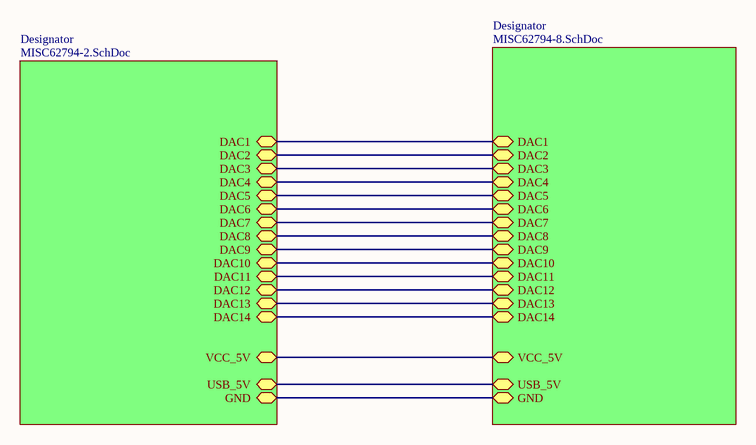
[diagram p0: MISC62794-10.SchDoc]
# Altium project MISC62794-12.PrjPcb (part 1 of 3)
3 sheets, 158 parts. Net scope: global (net labels, ports and power ports of the same name join across sheets).
Board file: MISC62794.PcbDoc
Sheets:
  MISC62794-10.SchDoc
    Designator = MISC62794-2.SchDoc
    Designator = MISC62794-8.SchDoc

## Sheet MISC62794-10.SchDoc
size A4

### Sub-sheets
Designator = MISC62794-2.SchDoc: DAC1 (bidir), DAC2 (bidir), DAC3 (bidir), DAC4 (bidir), DAC5 (bidir), DAC6 (bidir), DAC7 (bidir), DAC8 (bidir), DAC9 (bidir), DAC10 (bidir), DAC11 (bidir), DAC12 (bidir), DAC13 (bidir), DAC14 (bidir), USB_5V (bidir), GND (bidir), VCC_5V (bidir)
Designator = MISC62794-8.SchDoc: DAC1 (bidir), DAC2 (bidir), DAC3 (bidir), DAC4 (bidir), DAC5 (bidir), DAC6 (bidir), DAC7 (bidir), DAC8 (bidir), DAC9 (bidir), DAC10 (bidir), DAC11 (bidir), DAC12 (bidir), DAC13 (bidir), DAC14 (bidir), USB_5V (bidir), GND (bidir), VCC_5V (bidir)

### Nets
(unnamed): sheet Designator/DAC1, sheet Designator/DAC1
(unnamed): sheet Designator/DAC2, sheet Designator/DAC2
(unnamed): sheet Designator/DAC3, sheet Designator/DAC3
(unnamed): sheet Designator/DAC4, sheet Designator/DAC4
(unnamed): sheet Designator/DAC5, sheet Designator/DAC5
(unnamed): sheet Designator/DAC6, sheet Designator/DAC6
(unnamed): sheet Designator/DAC7, sheet Designator/DAC7
(unnamed): sheet Designator/DAC8, sheet Designator/DAC8
(unnamed): sheet Designator/DAC9, sheet Designator/DAC9
(unnamed): sheet Designator/DAC10, sheet Designator/DAC10
(unnamed): sheet Designator/DAC11, sheet Designator/DAC11
(unnamed): sheet Designator/DAC12, sheet Designator/DAC12
(unnamed): sheet Designator/DAC13, sheet Designator/DAC13
(unnamed): sheet Designator/DAC14, sheet Designator/DAC14
(unnamed): sheet Designator/USB_5V, sheet Designator/USB_5V
(unnamed): sheet Designator/GND, sheet Designator/GND
(unnamed): sheet Designator/VCC_5V, sheet Designator/VCC_5V

## Sheet MISC62794-2.SchDoc
size A4
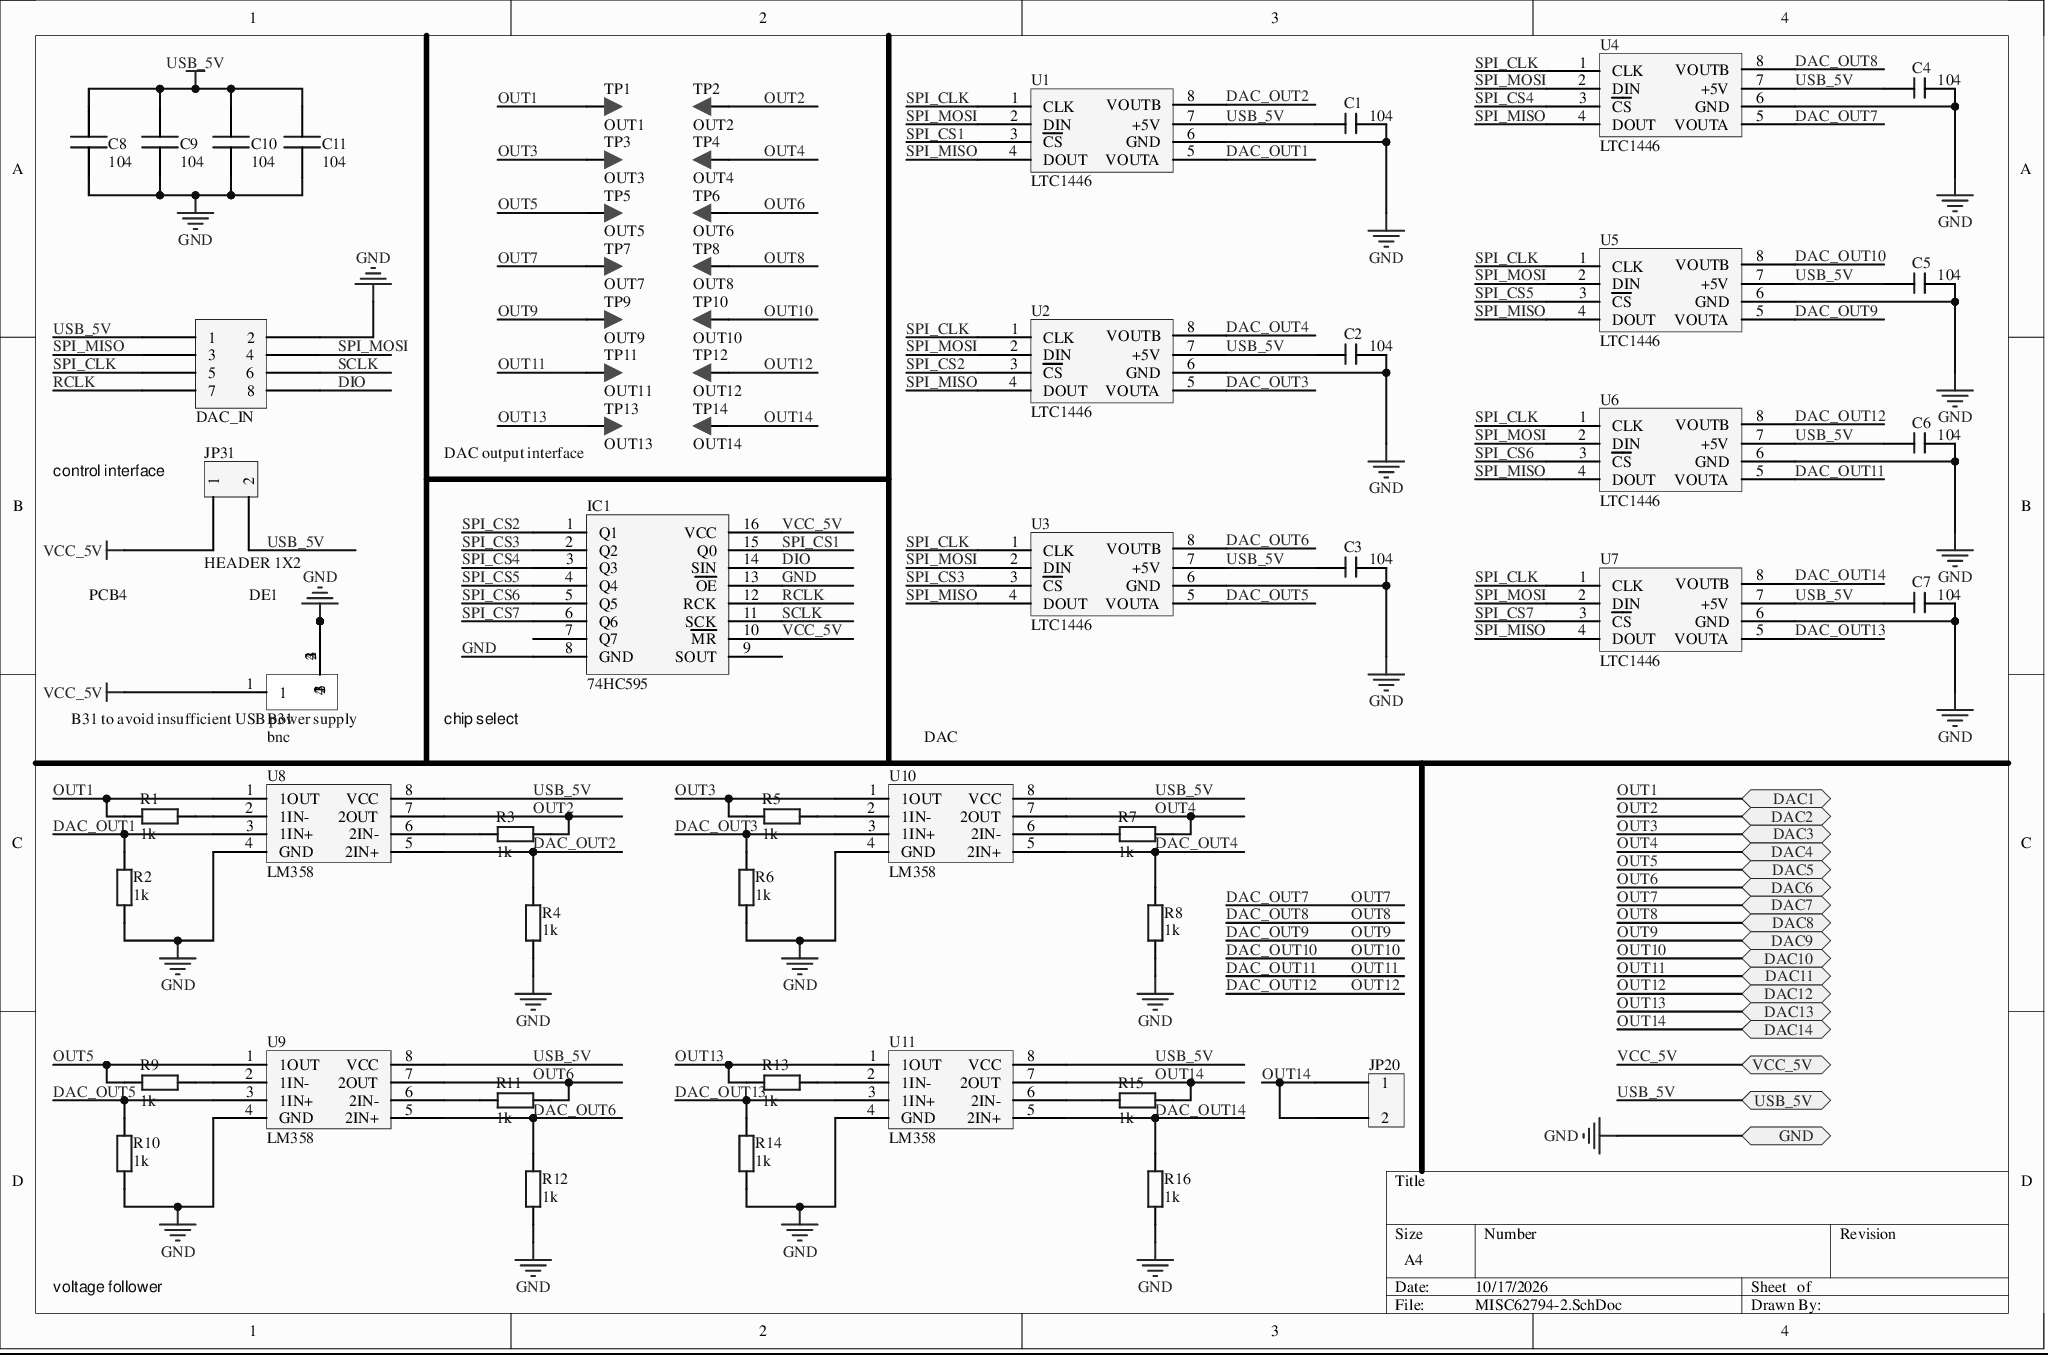
[diagram p1: MISC62794-2.SchDoc]

### Parts
B31  bnc  [BNC-TH_DOSIN-801-0072]
C1  104  [0603C]
C2  104  [0603C]
C3  104  [0603C]
C4  104  [0603C]
C5  104  [0603C]
C6  104  [0603C]
C7  104  [0603C]
C8  104  [0603C]
C9  104  [0603C]
C10  104  [0603C]
C11  104  [0603C]
DAC_IN  DAC_IN  [HDR2.54-LI-2x4P]  (value not drawn)
IC1  74HC595  [SOIC-16_L9.9-W3.9-P1.27-LS6.0-BL]
JP20  HEADER 1X2  [HDR2.54-LI-2P]  (value not drawn)
JP31  HEADER 1X2  [HDR2.54-LI-2P]
R1  1k  [0603R]
R2  1k  [0603R]
R3  1k  [0603R]
R4  1k  [0603R]
R5  1k  [0603R]
R6  1k  [0603R]
R7  1k  [0603R]
R8  1k  [0603R]
R9  1k  [0603R]
R10  1k  [0603R]
R11  1k  [0603R]
R12  1k  [0603R]
R13  1k  [0603R]
R14  1k  [0603R]
R15  1k  [0603R]
R16  1k  [0603R]
TP1  OUT1  [TP1.0]
TP2  OUT2  [TP1.0]
TP3  OUT3  [TP1.0]
TP4  OUT4  [TP1.0]
TP5  OUT5  [TP1.0]
TP6  OUT6  [TP1.0]
TP7  OUT7  [TP1.0]
TP8  OUT8  [TP1.0]
TP9  OUT9  [TP1.0]
TP10  OUT10  [TP1.0]
TP11  OUT11  [TP1.0]
TP12  OUT12  [TP1.0]
TP13  OUT13  [TP1.0]
TP14  OUT14  [TP1.0]
U1  LTC1446  [SO-8]
U2  LTC1446  [SO-8]
U3  LTC1446  [SO-8]
U4  LTC1446  [SO-8]
U5  LTC1446  [SO-8]
U6  LTC1446  [SO-8]
U7  LTC1446  [SO-8]
U8  LM358  [SO-8]
U9  LM358  [SO-8]
U10  LM358  [SO-8]
U11  LM358  [SO-8]

### Ports
DAC1 (bidir), DAC2 (bidir), DAC3 (bidir), DAC4 (bidir), DAC5 (bidir), DAC6 (bidir), DAC7 (bidir), DAC8 (bidir), DAC9 (bidir), DAC10 (bidir), DAC11 (bidir), DAC12 (bidir), DAC13 (bidir), DAC14 (bidir), GND (bidir), USB_5V (bidir), VCC_5V (bidir)

### Nets
GND: B31.2 B31.3 B31.4 C1.1 C2.1 C3.1 C4.1 C5.1 C6.1 C7.1 C8.2 C9.2 C10.2 C11.2 DAC_IN.2 IC1.8(GND) IC1.13(~{OE}) R2.2 R4.2 R6.2 R8.2 R10.2 R12.2 R14.2 R16.2 U1.6(GND) U2.6(GND) U3.6(GND) U4.6(GND) U5.6(GND) U6.6(GND) U7.6(GND) U8.4(GND) U9.4(GND) U10.4(GND) U11.4(GND) ; port GND
USB_5V: C1.2 C2.2 C3.2 C4.2 C5.2 C6.2 C7.2 C8.1 C9.1 C10.1 C11.1 DAC_IN.1 JP31.2 U1.7(+5V) U2.7(+5V) U3.7(+5V) U4.7(+5V) U5.7(+5V) U6.7(+5V) U7.7(+5V) U8.8(VCC) U9.8(VCC) U10.8(VCC) U11.8(VCC) ; port USB_5V
VCC_5V: B31.1 IC1.10(~{MR}) IC1.16(VCC) JP31.1 ; port VCC_5V
DAC_OUT1: R2.1 U1.5(VOUTA) U8.3(1IN+)
DAC_OUT2: R4.1 U1.8(VOUTB) U8.5(2IN+)
DAC_OUT3: R6.1 U2.5(VOUTA) U10.3(1IN+)
DAC_OUT4: R8.1 U2.8(VOUTB) U10.5(2IN+)
DAC_OUT5: R10.1 U3.5(VOUTA) U9.3(1IN+)
DAC_OUT6: R12.1 U3.8(VOUTB) U9.5(2IN+)
DAC_OUT7: TP7.1 U4.5(VOUTA) ; port DAC7  [also labelled OUT7]  [project net DAC7]
DAC_OUT8: TP8.1 U4.8(VOUTB) ; port DAC8  [also labelled OUT8]  [project net DAC8]
DAC_OUT9: TP9.1 U5.5(VOUTA) ; port DAC9  [also labelled OUT9]  [project net DAC9]
DAC_OUT10: TP10.1 U5.8(VOUTB) ; port DAC10  [also labelled OUT10]  [project net DAC10]
DAC_OUT11: TP11.1 U6.5(VOUTA) ; port DAC11  [also labelled OUT11]  [project net DAC11]
DAC_OUT12: TP12.1 U6.8(VOUTB) ; port DAC12  [also labelled OUT12]  [project net DAC12]
DAC_OUT13: R14.1 U7.5(VOUTA) U11.3(1IN+)
DAC_OUT14: R16.1 U7.8(VOUTB) U11.5(2IN+)
DIO: DAC_IN.8 IC1.14(SIN)
OUT1: R1.2 TP1.1 U8.1(1OUT) ; port DAC1  [project net DAC1]
OUT2: R3.1 TP2.1 U8.7(2OUT) ; port DAC2  [project net DAC2]
OUT3: R5.2 TP3.1 U10.1(1OUT) ; port DAC3  [project net DAC3]
OUT4: R7.1 TP4.1 U10.7(2OUT) ; port DAC4  [project net DAC4]
OUT5: R9.2 TP5.1 U9.1(1OUT) ; port DAC5  [project net DAC5]
OUT6: R11.1 TP6.1 U9.7(2OUT) ; port DAC6  [project net DAC6]
OUT13: R13.2 TP13.1 U11.1(1OUT) ; port DAC13  [project net DAC13]
OUT14: JP20.1 JP20.2 R15.1 TP14.1 U11.7(2OUT) ; port DAC14  [project net DAC14]
RCLK: DAC_IN.7 IC1.12(RCK)
SCLK: DAC_IN.6 IC1.11(SCK)
SPI_CLK: DAC_IN.5 U1.1(CLK) U2.1(CLK) U3.1(CLK) U4.1(CLK) U5.1(CLK) U6.1(CLK) U7.1(CLK)
SPI_CS1: IC1.15(Q0) U1.3(~{CS})
SPI_CS2: IC1.1(Q1) U2.3(~{CS})
SPI_CS3: IC1.2(Q2) U3.3(~{CS})
SPI_CS4: IC1.3(Q3) U4.3(~{CS})
SPI_CS5: IC1.4(Q4) U5.3(~{CS})
SPI_CS6: IC1.5(Q5) U6.3(~{CS})
SPI_CS7: IC1.6(Q6) U7.3(~{CS})
SPI_MISO: DAC_IN.3 U1.4(DOUT) U2.4(DOUT) U3.4(DOUT) U4.4(DOUT) U5.4(DOUT) U6.4(DOUT) U7.4(DOUT)
SPI_MOSI: DAC_IN.4 U1.2(DIN) U2.2(DIN) U3.2(DIN) U4.2(DIN) U5.2(DIN) U6.2(DIN) U7.2(DIN)
NetR1_1: R1.1 U8.2(1IN-)
NetR3_2: R3.2 U8.6(2IN-)
NetR5_1: R5.1 U10.2(1IN-)
NetR7_2: R7.2 U10.6(2IN-)
NetR9_1: R9.1 U9.2(1IN-)
NetR11_2: R11.2 U9.6(2IN-)
NetR13_1: R13.1 U11.2(1IN-)
NetR15_2: R15.2 U11.6(2IN-)

Not connected (* = marked no-connect by the designer): IC1 7(Q7) 9(SOUT)

### Notes on the sheet
- (near JP31) control interface
- (near TP13) DAC output interface
- PCB4
- DE1
- (near B31) B31 to avoid insufficient USB power supply
- chip select
- (near U10) DAC
- voltage follower

### Library data of the parts
C1-C11 = CAP: capacitor model
IC1 = 74HC595: IC
JP20 JP31 = HEADER 1X2: pin header
R1-R16 = RES: resistor model
TP1-TP14 = TP
U1-U7 = LTC1446: IC
U8-U11 = LM358: IC